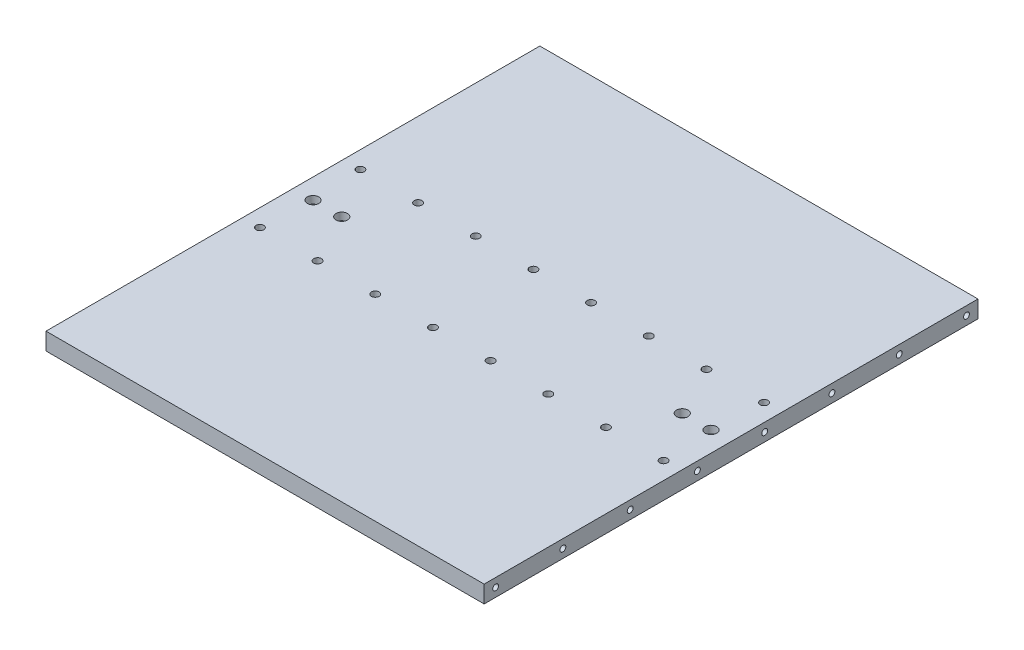
SolidWorks part; units mm, degrees
material "普通碳钢"
ref_plane "前视基准面" through (0, 0, 0) normal (0, 0, 1) x (1, 0, 0)
ref_plane "上视基准面" through (0, 0, 0) normal (0, 1, 0) x (1, 0, 0)
ref_plane "右视基准面" through (0, 0, 0) normal (1, 0, 0) x (0, 0, -1)
sketch "草图1" plane through (0, 0, 0) normal (0, 1, 0) x (1, 0, 0)
  line L1 (-381.5, -430) -> (381.5, -430)
  line L2 (-381.5, -430) -> (-381.5, 430)
  line L3 (-381.5, 430) -> (381.5, 430)
  line L4 (381.5, -430) -> (381.5, 430)
  line L5 (-381.5, -430) -> (381.5, 430) construction
  line L6 (-381.5, 430) -> (381.5, -430) construction
  point P0 (0, 0)
  dimension "D1" = 860
  dimension "D2" = 763
extrude "凸台-拉伸1" add sketch "草图1" along normal blind 30
hole_wizard "打孔尺寸(%根据)内六角圆柱头螺钉的类型1" positions "草图2" profile "草图3" counterbore size "M12" standard "GB" end condition through all
sketch "草图2" plane through (0, 0, 0) normal (0, -1, 0) x (-1, 0, 0)
  line L0 (-381.5, -430) -> (-381.5, 430) construction
  point P0 (351.5, 87.5)
  point P5 (351.5, -87.5)
  point P7 (251.0714, 87.5)
  point P9 (251.0714, -87.5)
  point P11 (150.6429, 87.5)
  point P13 (150.6429, -87.5)
  point P15 (50.2143, 87.5)
  point P17 (50.2143, -87.5)
  point P19 (-50.2143, -87.5)
  point P21 (-50.2143, 87.5)
  point P23 (-150.6429, 87.5)
  point P25 (-150.6429, -87.5)
  point P27 (-251.0714, 87.5)
  point P29 (-251.0714, -87.5)
  point P31 (-351.5, -87.5)
  point P33 (-351.5, 87.5)
  dimension "D1" = 30
  dimension "D2" = 130.4286
  dimension "D3" = 230.8571
  dimension "D4" = 331.2857
  dimension "D5" = 431.7143
  dimension "D6" = 532.1429
  dimension "D7" = 632.5714
  dimension "D8" = 733
  dimension "D9" = 342.5
  dimension "D10" = 517.5
sketch "草图3" plane through (-351.5, 0, -87.5) normal (1, 0, 0) x (0, 0, -1)
  line L0 (0, 0) -> (0, 30)
  line L1 (0, 30) -> (6.75, 30)
  line L3 (6.75, 30) -> (6.75, 13)
  line L4 (6.75, 13) -> (10, 13)
  line L5 (10, 13) -> (10, 0)
  line L7 (10, 0) -> (0, 0)
  line L11 (0, -6.35) -> (0, 107.95) construction
  dimension "通孔孔直径" = 13.5
  dimension "通孔孔深度" = 30
  dimension "柱形沉头孔直径" = 20
  dimension "柱形沉头孔深度" = 13
hole_wizard "打孔尺寸(%根据)内六角圆柱头螺钉的类型2" positions "草图4" profile "草图5" counterbore size "M12" standard "GB" end condition through all
sketch "草图4" plane through (0, 30, 0) normal (0, 1, 0) x (1, 0, 0)
  circle A0 centre (-351.5, 87.5) radius 6.75 construction
  point P0 (-346.5, 0)
  point P2 (-296.5, 0)
  point P4 (346.5, 0)
  point P6 (296.5, 0)
  dimension "D1" = 5
  dimension "D2" = 55
  dimension "D3" = 648
  dimension "D4" = 698
  dimension "D5" = 87.5
sketch "草图5" plane through (-346.5, 30, 0) normal (1, 0, 0) x (0, 0, 1)
  line L0 (0, 0) -> (0, 30)
  line L1 (0, 30) -> (6.75, 30)
  line L3 (6.75, 30) -> (6.75, 13)
  line L4 (6.75, 13) -> (10, 13)
  line L5 (10, 13) -> (10, 0)
  line L7 (10, 0) -> (0, 0)
  line L11 (0, -6.35) -> (0, 107.95) construction
  dimension "通孔孔直径" = 13.5
  dimension "通孔孔深度" = 30
  dimension "柱形沉头孔直径" = 20
  dimension "柱形沉头孔深度" = 13
hole_wizard "M12 螺纹孔1" positions "草图6" profile "草图7" tap size "M12" standard "GB"
sketch "草图6" plane through (-381.5, 0, 0) normal (-1, 0, 0) x (0, 0, 1)
  line L0 (430, 30) -> (430, 0) construction
  line L1 (-430, 30) -> (-430, 0) construction
  line L2 (-410, 15) -> (-292.8571, 15) construction
  line L3 (-292.8571, 15) -> (-175.7143, 15) construction
  line L4 (-175.7143, 15) -> (-58.5714, 15) construction
  line L5 (-58.5714, 15) -> (58.5714, 15) construction
  line L6 (58.5714, 15) -> (175.7143, 15) construction
  line L7 (175.7143, 15) -> (292.8571, 15) construction
  line L8 (292.8571, 15) -> (410, 15) construction
  point P0 (410, 15)
  point P2 (292.8571, 15)
  point P4 (175.7143, 15)
  point P6 (58.5714, 15)
  point P8 (-58.5714, 15)
  point P10 (-175.7143, 15)
  point P12 (-292.8571, 15)
  point P14 (-410, 15)
  point P21 (430, 15)
  dimension "D1" = 20
  dimension "D2" = 20
sketch "草图7" plane through (-381.5, 15, 410) normal (0, 1, 0) x (0, 0, 1)
  line L0 (0, 0) -> (0, 32.3144)
  line L1 (0, 32.3144) -> (5.1, 29.25)
  line L2 (5.1, 29.25) -> (5.1, 0)
  line L5 (5.1, 0) -> (0, 0)
  line L10 (0, 32.3144) -> (-5.1, 29.25) construction
  line L11 (0, -6.35) -> (0, 107.95) construction
  dimension "螺纹孔钻头直径" = 10.2
  dimension "螺纹孔钻头深度" = 29.25
  dimension "导头角度" = 118
cosmetic thread "孔螺蚊线1"
cosmetic thread "孔螺蚊线2"
cosmetic thread "孔螺蚊线3"
cosmetic thread "孔螺蚊线4"
cosmetic thread "孔螺蚊线5"
cosmetic thread "孔螺蚊线6"
cosmetic thread "孔螺蚊线7"
cosmetic thread "孔螺蚊线8"
hole_wizard "M12 螺纹孔2" positions "草图8" profile "草图9" tap size "M12" standard "GB"
sketch "草图8" plane through (381.5, 0, 0) normal (1, 0, 0) x (0, 0, -1)
  line L0 (430, 30) -> (430, 0) construction
  line L1 (-430, 0) -> (430, 0) construction
  point P0 (-410, 15)
  point P2 (-292.8571, 15)
  point P4 (-175.7143, 15)
  point P6 (-58.5714, 15)
  point P8 (58.5714, 15)
  point P10 (175.7143, 15)
  point P12 (292.8571, 15)
  point P14 (410, 15)
  dimension "D1" = 20
  dimension "D2" = 137.1429
  dimension "D3" = 254.2857
  dimension "D4" = 371.4286
  dimension "D5" = 488.5714
  dimension "D6" = 605.7143
  dimension "D7" = 722.8571
  dimension "D8" = 840
  dimension "D9" = 15
sketch "草图9" plane through (381.5, 15, 410) normal (0, 1, 0) x (0, 0, -1)
  line L0 (0, 0) -> (0, 32.3144)
  line L1 (0, 32.3144) -> (5.1, 29.25)
  line L2 (5.1, 29.25) -> (5.1, 0)
  line L5 (5.1, 0) -> (0, 0)
  line L10 (0, 32.3144) -> (-5.1, 29.25) construction
  line L11 (0, -6.35) -> (0, 107.95) construction
  dimension "螺纹孔钻头直径" = 10.2
  dimension "螺纹孔钻头深度" = 29.25
  dimension "导头角度" = 118
cosmetic thread "孔螺蚊线9"
cosmetic thread "孔螺蚊线10"
cosmetic thread "孔螺蚊线11"
cosmetic thread "孔螺蚊线12"
cosmetic thread "孔螺蚊线13"
cosmetic thread "孔螺蚊线14"
cosmetic thread "孔螺蚊线15"
cosmetic thread "孔螺蚊线16"
